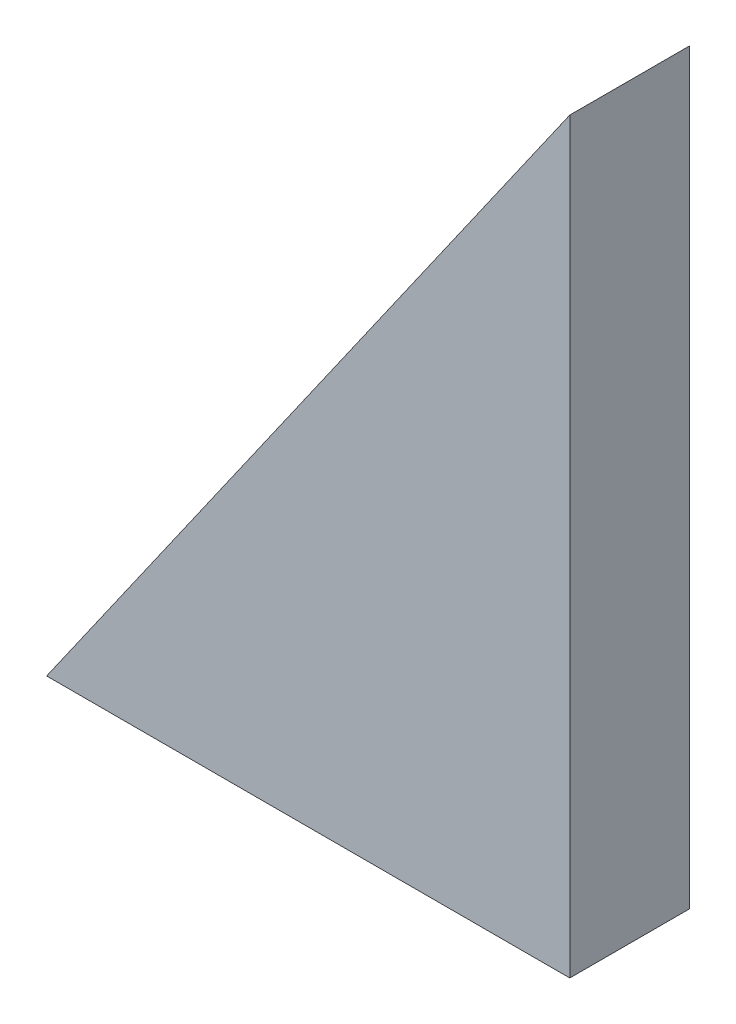
SolidWorks part; units mm, degrees
material "A3"
ref_plane "前视基准面" through (0, 0, 0) normal (0, 0, 1) x (1, 0, 0)
ref_plane "上视基准面" through (0, 0, 0) normal (0, 1, 0) x (1, 0, 0)
ref_plane "右视基准面" through (0, 0, 0) normal (1, 0, 0) x (0, 0, -1)
sketch "草图1" plane through (0, 0, 0) normal (0, 0, 1) x (1, 0, 0)
  line L0 (0, 0) -> (35, 0)
  line L1 (35, 0) -> (35, 50)
  line L2 (35, 50) -> (0, 0)
  dimension "D1" = 35
  dimension "D2" = 50
extrude "凸台-拉伸1" add sketch "草图1" along normal mid plane 8
